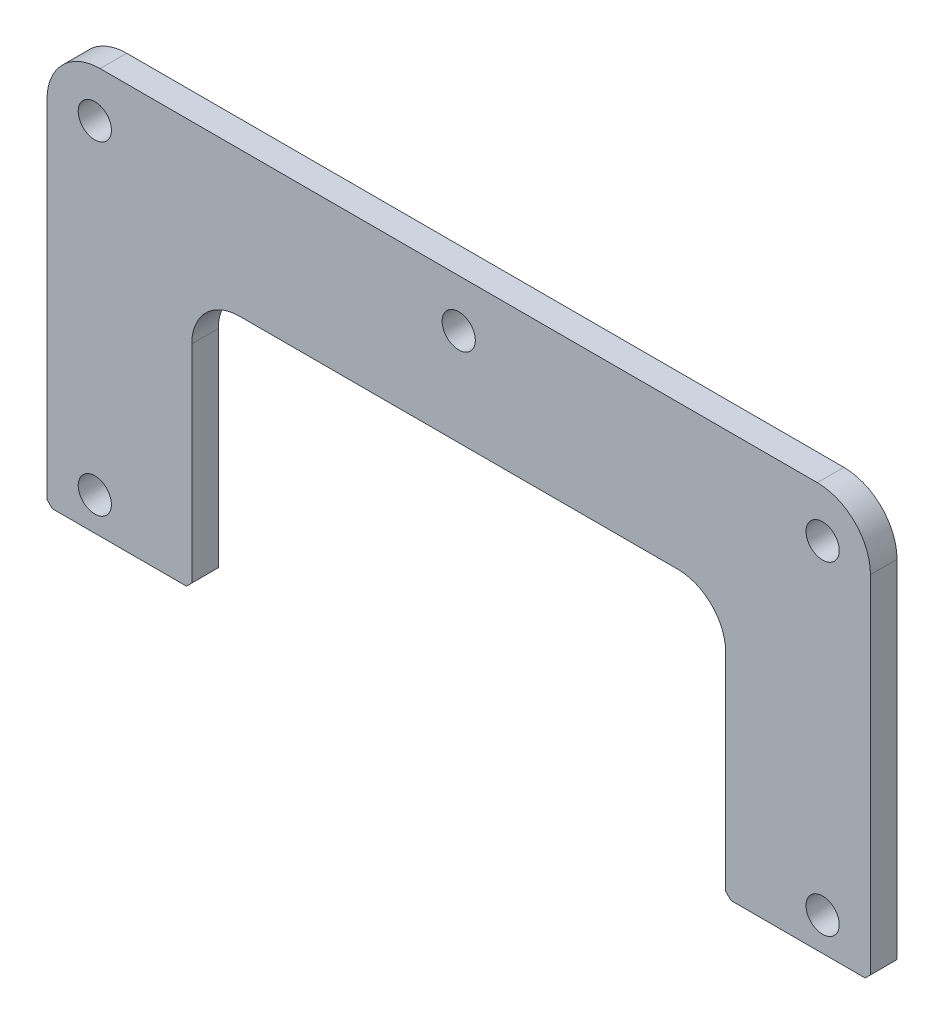
from build123d import *

# Parameters (mm, degrees)
EXTRUDE_1_DEPTH     = 10
SKETCH_2_R          = 6.25
CUT_EXTRUDE_1_DEPTH = 220.431082575
CHAMFER_1_SIZE      = 2


with BuildPart() as part:
    # 草图1 → 凸台-拉伸1 (new body)
    with BuildSketch(Plane.XY):
        with BuildLine():
            Line((-82.5, 100.5), (82.5, 100.5))
            ThreePointArc((82.5, 100.5), (95.227922061, 95.227922061), (100.5, 82.5))
            Line((100.5, 82.5), (100.5, 2.5))
            Line((100.5, 2.5), (155, 2.5))
            Line((155, 2.5), (155, 135))
            ThreePointArc((155, 135), (149.142135624, 149.142135624), (135, 155))
            Line((135, 155), (-135, 155))
            ThreePointArc((-135, 155), (-149.142135624, 149.142135624), (-155, 135))
            Line((-155, 135), (-155, 2.5))
            Line((-155, 2.5), (-100.5, 2.5))
            Line((-100.5, 2.5), (-100.5, 82.5))
            ThreePointArc((-100.5, 82.5), (-95.227922061, 95.227922061), (-82.5, 100.5))
        make_face()
    extrude(amount=EXTRUDE_1_DEPTH)

    # 草图2 → 切除-拉伸1 (cut, through all)
    with BuildSketch(Plane.XY.offset(10)):
        with Locations((0, 137)):
            Circle(SKETCH_2_R)
        with Locations((0, -137)):
            Circle(SKETCH_2_R)
        with Locations((-137, 137)):
            Circle(SKETCH_2_R)
        with Locations((137, 137)):
            Circle(SKETCH_2_R)
        with Locations((-137, -137)):
            Circle(SKETCH_2_R)
        with Locations((137, -137)):
            Circle(SKETCH_2_R)
        with Locations((-137, 15)):
            Circle(SKETCH_2_R)
        with Locations((-137, -15)):
            Circle(SKETCH_2_R)
        with Locations((137, -15)):
            Circle(SKETCH_2_R)
        with Locations(Location((137, 15, 0), (0, 0, 180))):
            Circle(SKETCH_2_R)
    extrude(amount=-CUT_EXTRUDE_1_DEPTH, mode=Mode.SUBTRACT)

    # 倒角1
    chamfer_1_edges = [part.edges().sort_by_distance(p)[0] for p in [
        (-100.5, 2.5, 5),
        (-155, 2.5, 5),
        (155, 2.5, 5),
        (100.5, 2.5, 5),
    ]]
    chamfer(chamfer_1_edges, length=CHAMFER_1_SIZE)


solid = part.part
